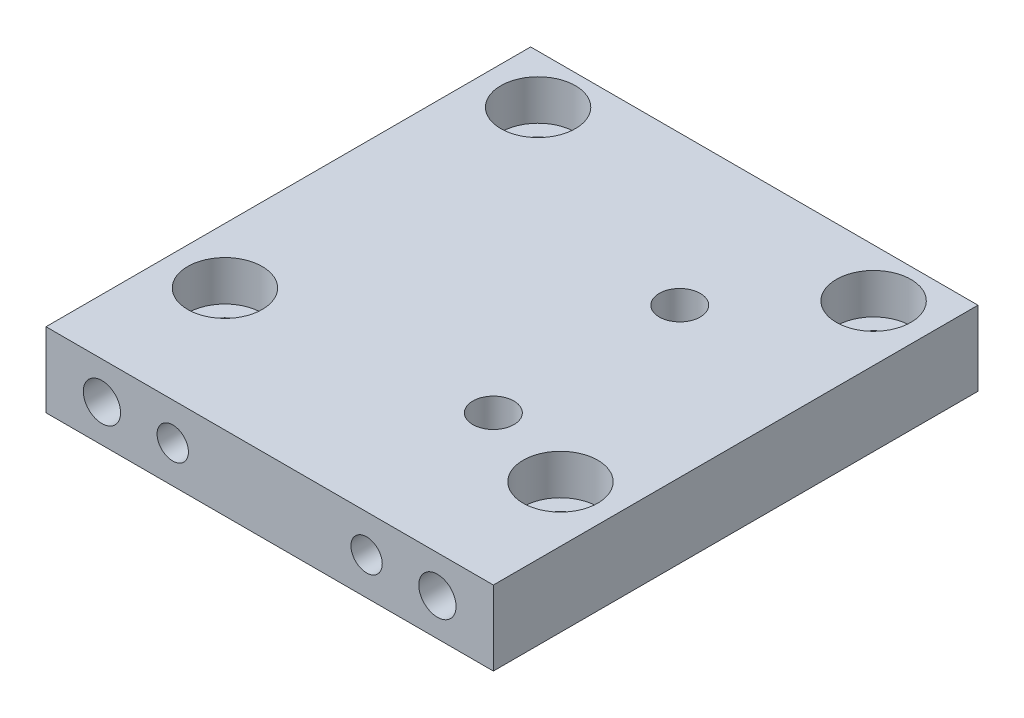
SolidWorks part; units mm, degrees
material "AL6061"
ref_plane "前视基准面" through (0, 0, 0) normal (0, 0, 1) x (1, 0, 0)
ref_plane "上视基准面" through (0, 0, 0) normal (0, 1, 0) x (1, 0, 0)
ref_plane "右视基准面" through (0, 0, 0) normal (1, 0, 0) x (0, 0, -1)
sketch "草图1" plane through (0, 0, 0) normal (0, 1, 0) x (1, 0, 0)
  line L1 (-30, 32.5) -> (30, 32.5)
  line L2 (-30, 32.5) -> (-30, -32.5)
  line L3 (-30, -32.5) -> (30, -32.5)
  line L4 (30, 32.5) -> (30, -32.5)
  line L5 (-30, 32.5) -> (30, -32.5) construction
  line L6 (-30, -32.5) -> (30, 32.5) construction
  point P0 (0, 0)
  dimension "D1" = 60
  dimension "D2" = 65
extrude "凸台-拉伸1" add sketch "草图1" along normal mid plane 10
sketch "草图2" plane through (0, 5, 0) normal (0, 1, 0) x (1, 0, 0)
  point P0 (-22.5, 26)
  point P3 (-22.5, -16)
  point P6 (22.5, -16)
  point P9 (22.5, 26)
hole_wizard "M5 六角凹头螺钉的柱形沉头孔1" positions "草图2" profile "草图3" counterbore size "M5" standard "ISO" end condition through all
sketch "草图3" plane through (-22.5, 5, -26) normal (1, 0, 0) x (0, 0, 1)
  line L0 (0, 0) -> (0, 10)
  line L1 (0, 10) -> (2.75, 10)
  line L3 (2.75, 10) -> (2.75, 5.4)
  line L4 (2.75, 5.4) -> (5, 5.4)
  line L5 (5, 5.4) -> (5, 0)
  line L7 (5, 0) -> (0, 0)
  line L11 (0, -6.35) -> (0, 107.95) construction
  dimension "通孔孔直径" = 5.5
  dimension "通孔孔深度" = 10
  dimension "柱形沉头孔直径" = 10
  dimension "柱形沉头孔深度" = 5.4
hole_wizard "Ø5.0mm 暗销孔1" positions "草图4" profile "草图5" hole size "Ø5.0" standard "ISO"
sketch "草图4" plane through (0, 0, 32.5) normal (0, 0, 1) x (1, 0, 0)
  line L0 (0, 0) -> (0, -15.9204) construction
  line L1 (-30, 5) -> (-30, -5) construction
  point P0 (-22.5, 0)
  point P10 (22.5, 0)
  dimension "D1" = 7.5
sketch "草图5" plane through (-22.5, 0, 32.5) normal (1, 0, 0) x (0, -1, 0)
  line L0 (0, 0) -> (0, 7)
  line L1 (0, 7) -> (2.5, 7)
  line L2 (2.5, 7) -> (2.5, 0)
  line L5 (2.5, 0) -> (0, 0)
  line L10 (0, 7) -> (-2.5, 7) construction
  line L11 (0, -6.35) -> (0, 107.95) construction
  dimension "孔直径" = 5
  dimension "孔深度" = 7
  dimension "导头角度" = 180
sketch "草图6" plane through (0, 0, 32.5) normal (0, 0, 1) x (1, 0, 0)
  line L0 (-30, 5) -> (-30, -5) construction
  line L1 (0, 0) -> (0, 10.6669) construction
  point P0 (-13, 0)
  point P12 (13, 0)
  dimension "D1" = 17
hole_wizard "M5 螺纹孔1" positions "草图6" profile "草图7" tap size "M5" standard "ISO"
sketch "草图7" plane through (-13, 0, 32.5) normal (1, 0, 0) x (0, -1, 0)
  line L0 (0, 0) -> (0, 13.6618)
  line L1 (0, 13.6618) -> (2.1, 12.4)
  line L2 (2.1, 12.4) -> (2.1, 0)
  line L5 (2.1, 0) -> (0, 0)
  line L10 (0, 13.6618) -> (-2.1, 12.4) construction
  line L11 (0, -6.35) -> (0, 107.95) construction
  dimension "螺纹孔钻头直径" = 4.2
  dimension "螺纹孔钻头深度" = 12.4
  dimension "导头角度" = 118
cosmetic thread "孔螺蚊线1" parameters "D1"=10, "D2"=5
cosmetic thread "孔螺蚊线2" parameters "D1"=10, "D2"=5
sketch "草图8" plane through (0, -5, 0) normal (0, -1, 0) x (-1, 0, 0)
  point P0 (-10, -12.5)
  point P3 (-10, 12.5)
hole_wizard "M5 六角凹头螺钉的柱形沉头孔2" positions "草图8" profile "草图9" counterbore size "M5" standard "ISO" end condition through all
sketch "草图9" plane through (10, -5, 12.5) normal (1, 0, 0) x (0, 0, -1)
  line L0 (0, 0) -> (0, 10)
  line L1 (0, 10) -> (2.75, 10)
  line L3 (2.75, 10) -> (2.75, 5.4)
  line L4 (2.75, 5.4) -> (5, 5.4)
  line L5 (5, 5.4) -> (5, 0)
  line L7 (5, 0) -> (0, 0)
  line L11 (0, -6.35) -> (0, 107.95) construction
  dimension "通孔孔直径" = 5.5
  dimension "通孔孔深度" = 10
  dimension "柱形沉头孔直径" = 10
  dimension "柱形沉头孔深度" = 5.4
